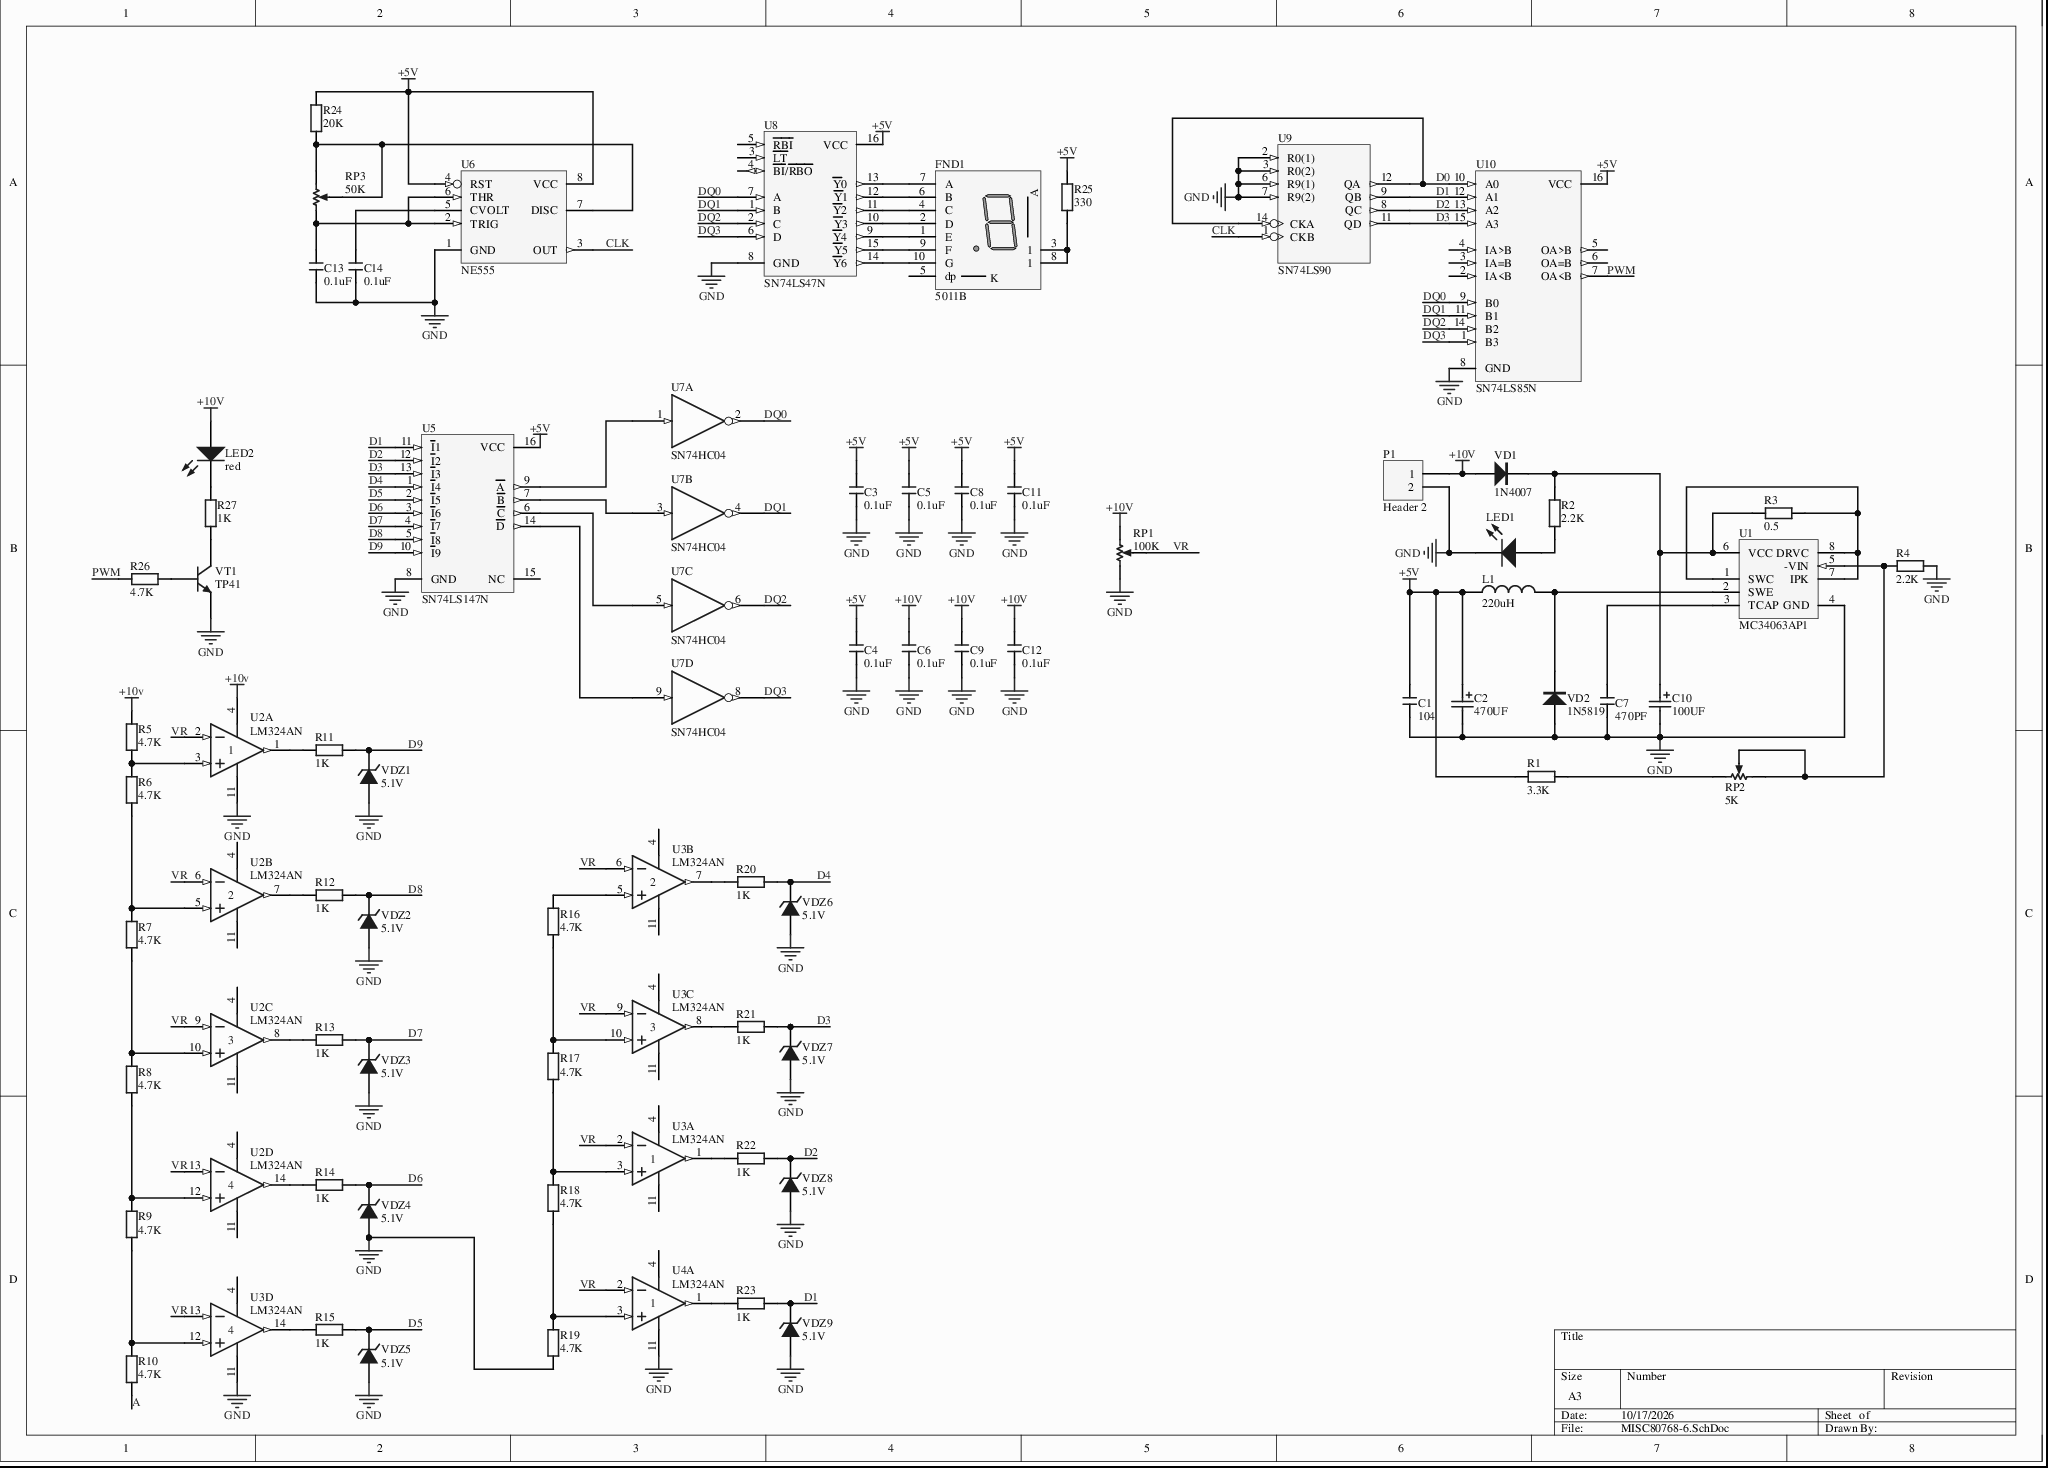
[diagram p0: MISC80768-6.SchDoc]
# Altium project MISC80768-2.PrjPcb
1 sheet, 71 parts. Net scope: global (net labels, ports and power ports of the same name join across sheets).
Board file: MISC80768.PcbDoc

## Sheet MISC80768-6.SchDoc
size A3

### Parts
C1  104  [CC 2.2*5]
C2  470UF  [CAP 1.5*4*8]
C3  0.1uF  [CC 2.2*5]
C4  0.1uF  [CC 2.2*5]
C5  0.1uF  [CC 2.2*5]
C6  0.1uF  [CC 2.2*5]
C7  470PF  [CC 2.2*5]
C8  0.1uF  [CC 2.2*5]
C9  0.1uF  [CC 2.2*5]
C10  100UF  [CAP 1.5*4*8]
C11  0.1uF  [CC 2.2*5]
C12  0.1uF  [CC 2.2*5]
C13  0.1uF  [CC 2.2*5]
C14  0.1uF  [CC 2.2*5]
FND1  5011B  [SMG 0.5-1P]
L1  220uH  [AL0307]
LED1  red  [LED 3MM-B]  (value not drawn)
LED2  red  [LED 3MM-B]
P1  Header 2  [HDR1X2]
R1  3.3K  [RS 1/4W]
R2  2.2K  [RS 1/4W]
R3  0.5  [RS 1/4W]
R4  2.2K  [RS 1/4W]
R5  4.7K  [RS 1/4W]
R6  4.7K  [RS 1/4W]
R7  4.7K  [RS 1/4W]
R8  4.7K  [RS 1/4W]
R9  4.7K  [RS 1/4W]
R10  4.7K  [RS 1/4W]
R11  1K  [RS 1/4W]
R12  1K  [RS 1/4W]
R13  1K  [RS 1/4W]
R14  1K  [RS 1/4W]
R15  1K  [RS 1/4W]
R16  4.7K  [RS 1/4W]
R17  4.7K  [RS 1/4W]
R18  4.7K  [RS 1/4W]
R19  4.7K  [RS 1/4W]
R20  1K  [RS 1/4W]
R21  1K  [RS 1/4W]
R22  1K  [RS 1/4W]
R23  1K  [RS 1/4W]
R24  20K  [RS 1/4W]
R25  330  [RS 1/4W]
R26  4.7K  [RS 1/4W]
R27  1K  [RS 1/4W]
RP1  100K  [VR5]
RP2  5K  [VR5]
RP3  50K  [VR5]
U1  MC34063AP1  [626-05]
U2  LM324AN  [646-06]  (parts A,B,C,D of 4)
U3  LM324AN  [646-06]  (parts A,B,C,D of 4)
U4  LM324AN  [646-06]  (part A of 4)
U5  SN74LS147N  [648-08]
U6  NE555  [DIP8]
U7  SN74HC04  [SO14]  (parts A,B,C,D of 6)
U8  SN74LS47N  [648-08]
U9  SN74LS90  [DIP14]
U10  SN74LS85N  [648-08]
VD1  1N4007  [DO-41]
VD2  1N5819  [DO-41]
VDZ1  5.1V  [DO-35]
VDZ2  5.1V  [DO-35]
VDZ3  5.1V  [DO-35]
VDZ4  5.1V  [DO-35]
VDZ5  5.1V  [DO-35]
VDZ6  5.1V  [DO-35]
VDZ7  5.1V  [DO-35]
VDZ8  5.1V  [DO-35]
VDZ9  5.1V  [DO-35]
VT1  TP41  [TO-92A]

### Nets
+5V: C1.1 C2.1 C3.1 C4.1 C5.1 C8.1 C11.1 L1.1 R1.2 R24.2 R25.2 U5.16(VCC) U6.4(RST) U6.8(VCC) U8.16(VCC) U10.16(VCC)
+10V: C6.1 C9.1 C12.1 LED2.1(A) P1.1 R5.1 RP1.2(BOT) U2.4(V+) VD1.1(A)
GND: C1.2 C2.2 C3.2 C4.2 C5.2 C6.2 C7.2 C8.2 C9.2 C10.2 C11.2 C12.2 C13.2 C14.2 LED1.2(K) P1.2 R4.1 R19.2 RP1.1(TOP) U1.4(GND) U2.11(V-) U3.11(V-) U4.11(V-) U5.8(GND) U6.1(GND) U7.7(GND) U8.8(GND) U9.2(R0(1)) U9.3(R0(2)) U9.6(R9(1)) U9.7(R9(2)) U9.10(GND) U10.8(GND) VD2.1(A) VDZ1.1(A) VDZ2.1(A) VDZ3.1(A) VDZ4.1(A) VDZ5.1(A) VDZ6.1(A) VDZ7.1(A) VDZ8.1(A) VDZ9.1(A) VT1.1(E)
VCC: U7.14(VCC) U9.5(VCC)
A: R10.2
CLK: U6.3(OUT) U9.1(CKB)
D0: U9.12(QA) U9.14(CKA) U10.10(A0)
D1: R23.2 U5.11(~{I}1) U9.9(QB) U10.12(A1) VDZ9.2(K)
D2: R22.2 U5.12(~{I}2) U9.8(QC) U10.13(A2) VDZ8.2(K)
D3: R21.2 U5.13(~{I}3) U9.11(QD) U10.15(A3) VDZ7.2(K)
D4: R20.2 U5.1(~{I}4) VDZ6.2(K)
D5: R15.2 U5.2(~{I}5) VDZ5.2(K)
D6: R14.2 U5.3(~{I}6) VDZ4.2(K)
D7: R13.2 U5.4(~{I}7) VDZ3.2(K)
D8: R12.2 U5.5(~{I}8) VDZ2.2(K)
D9: R11.2 U5.10(~{I}9) VDZ1.2(K)
DQ0: U7.2 U8.7(A) U10.9(B0)
DQ1: U7.4 U8.1(B) U10.11(B1)
DQ2: U7.6 U8.2(C) U10.14(B2)
DQ3: U7.8 U8.6(D) U10.1(B3)
PWM: R26.2 U10.7(OA<B)
VR: RP1.3(TAP) U2.2(IN-) U2.6(IN-) U2.9(IN-) U2.13(IN-) U3.2(IN-) U3.6(IN-) U3.9(IN-) U3.13(IN-) U4.2(IN-)
NetC7_1: C7.1 U1.3(TCAP)
NetC10_1: C10.1 R2.2 R3.2 U1.6(VCC) VD1.2(K)
NetC13_1: C13.1 RP3.1(TOP) U6.2(TRIG) U6.6(THR)
NetC14_1: C14.1 U6.5(CVOLT)
NetFND1_1: FND1.1(E) U8.9(~{Y}4)
NetFND1_2: FND1.2(D) U8.10(~{Y}3)
NetFND1_3: FND1.3(1) FND1.8(1) R25.1
NetFND1_4: FND1.4(C) U8.11(~{Y}2)
NetFND1_6: FND1.6(B) U8.12(~{Y}1)
NetFND1_7: FND1.7(A) U8.13(~{Y}0)
NetFND1_9: FND1.9(F) U8.15(~{Y}5)
NetFND1_10: FND1.10(G) U8.14(~{Y}6)
NetL1_2: L1.2 U1.2(SWE) VD2.2(K)
NetLED1_1: LED1.1(A) R2.1
NetLED2_2: LED2.2(K) R27.2
NetR1_1: R1.1 RP2.2(BOT)
NetR3_1: R3.1 U1.1(SWC) U1.7(IPK) U1.8(DRVC)
NetR4_2: R4.2 RP2.1(TOP) RP2.3(TAP) U1.5(-VIN)
NetR5_2: R5.2 R6.1 U2.3(IN+)
NetR6_2: R6.2 R7.1 U2.5(IN+)
NetR7_2: R7.2 R8.1 U2.10(IN+)
NetR8_2: R8.2 R9.1 U2.12(IN+)
NetR9_2: R9.2 R10.1 U3.12(IN+)
NetR11_1: R11.1 U2.1(OUT)
NetR12_1: R12.1 U2.7(OUT)
NetR13_1: R13.1 U2.8(OUT)
NetR14_1: R14.1 U2.14(OUT)
NetR15_1: R15.1 U3.14(OUT)
NetR16_1: R16.1 U3.5(IN+)
NetR16_2: R16.2 R17.1 U3.10(IN+)
NetR17_2: R17.2 R18.1 U3.3(IN+)
NetR18_2: R18.2 R19.1 U4.3(IN+)
NetR20_1: R20.1 U3.7(OUT)
NetR21_1: R21.1 U3.8(OUT)
NetR22_1: R22.1 U3.1(OUT)
NetR23_1: R23.1 U4.1(OUT)
NetR24_1: R24.1 RP3.2(BOT) RP3.3(TAP) U6.7(DISC)
NetR26_1: R26.1 VT1.2(B)
NetR27_1: R27.1 VT1.3(C)
NetU5_6: U5.6(~{C}) U7.5
NetU5_7: U5.7(~{B}) U7.3
NetU5_9: U5.9(~{A}) U7.1
NetU5_14: U5.14(~{D}) U7.9

Not connected (* = marked no-connect by the designer): FND1 5(dp)*; U3 4(V+); U4 4(V+); U5 15(NC)*; U8 3(~{LT})* 4(~{BI}/~{RBO})* 5(~{RBI})*; U10 2(IA<B)* 3(IA=B)* 4(IA>B)* 5(OA>B)* 6(OA=B)*

### Library data of the parts
C1 C3-C9 C11-C14 = CC: ceramic capacitor; BOM名称: through-hole ceramic capacitor
C2 C10 = Cap Pol2: Polarized Capacitor (Axial); Value: 100pF; Published: 8-Jun-2000; LatestRevisionDate: 17-Jul-2002; LatestRevisionNote: Re-released for DXP Platform.; PackageReference: POLAR0.8; PackageDescription: Polarized Capacitor; 2 Leads; Publisher: Altium Limited
FND1 = 5011B: 0.5 inch 1-digit common-anode seven-segment display; BOM名称: 0.5 inch 1-digit common-anode
L1 = L-AL: color-band inductor; BOM名称: color-band inductor
LED1 LED2 = LED-3MM: 3mm through-hole LED; BOM名称: through-hole LED
P1 = Header 2: Header, 2-Pin; LatestRevisionDate: 17-Jul-2002; LatestRevisionNote: Re-released for DXP Platform.; Publisher: Altium Limited
R1-R27 = R-S: color-band resistor; BOM名称: color-band resistor
RP1-RP3 = RPot: Potentiometer; Sim Note: Enter the Resistance value and the set point into parameter fields.; Set Position: 0.5; Value: 1K; Published: 8-Jun-2000; LatestRevisionDate: 17-Jul-2002; LatestRevisionNote: Re-released for DXP Platform.; PackageReference: VR5; PackageDescription: Variable Resistor, Thru-Hole; 3 Leads; Publisher: Altium Limited
U1 = MC34063AP1: DC-to-DC Converter Control Circuit; Published: 17-Jul-2002; Datasheet: Linear and Interface Integrated Circuits, DL128 Rev2 (1988); Package Reference: 626-05; Publisher: Altium Limited
U2-U4 = LM324AN: Quad Low-Power Operational Amplifier; Package Information: Latest Revision: 1997; Published: 17-Jul-2002; Datasheet: Linear and Interface Integrated Circuits, DL128 Rev2 (1988); Package Reference: 646-06; Publisher: Altium Limited
U5 = SN74LS147N: 10-Line-to-4-Line Priority Encoder; Package Information: Latest Revision: Apr-2000; Code - JEDEC: MS-001-BB; Published: 15-Apr-2002; Datasheet: Latest Revision: Dec-1999; Package Reference: 648-08; Publisher: Altium Limited
U6 = NE555D: General-Purpose Single Bipolar Timer; Package Information: Latest Revision: Jul-1998; Code - JEDEC: MS-012-AA; Code - IPC: SO8; Published: 24-Aug-2001; Revision: 17-Jul-2002: Re-released for DXP Platform.; Datasheet: Latest Revision: Jul-1998; Package Reference: SO8; Publisher: Altium Limited
U7 = SN74HC04: Hex Inverters
U8 = SN74LS47N: BCD to 7-Segment Decoder/Driver; Package Information: Latest Revision: Apr-2000; Code - JEDEC: MS-001-BB; Published: 15-Apr-2002; Datasheet: Latest Revision: Dec-1999; Package Reference: 648-08; Publisher: Altium Limited
U9 = SN74LS90: DECADE DIV-BY-12 BIN CNT
U10 = SN74LS85N: 4-Bit Magnitude Comparator; Package Information: Latest Revision: Apr-2000; Code - JEDEC: MS-001-BB; Published: 15-Apr-2002; Datasheet: Latest Revision: Dec-1999; Package Reference: 648-08; Publisher: Altium Limited
VD1 VD2 = 1N4007: rectifier diode; BOM名称: rectifier diode
VDZ1-VDZ9 = 1N4619: 3V/0.5W zener diode; BOM名称: 3V/0.5W zener diode
VT1 = 2N3904: NPN General Purpose Amplifier; Published: 8-Jun-2000; LatestRevisionDate: 15-Jan-2003; LatestRevisionNote: PCB Footprint 'BCY-W3/D4.7' replaced; DatasheetVersion: 1997; PackageVersion: Sep-1998; PackageReference: TO-92A; PackageDescription: TO, Flat Index; 3 In-Line, Axial Leads; Body Dia. 4.5mm; Leads 0.51 x 0.48 mm (max); ComponentLink1Description: Manufacturer Link; ComponentLink2Description: Datasheet; ComponentLink2URL: http://www.fairchildsemi.com/ds/2N%2F2N3904.pdf; Publisher: Altium Limited